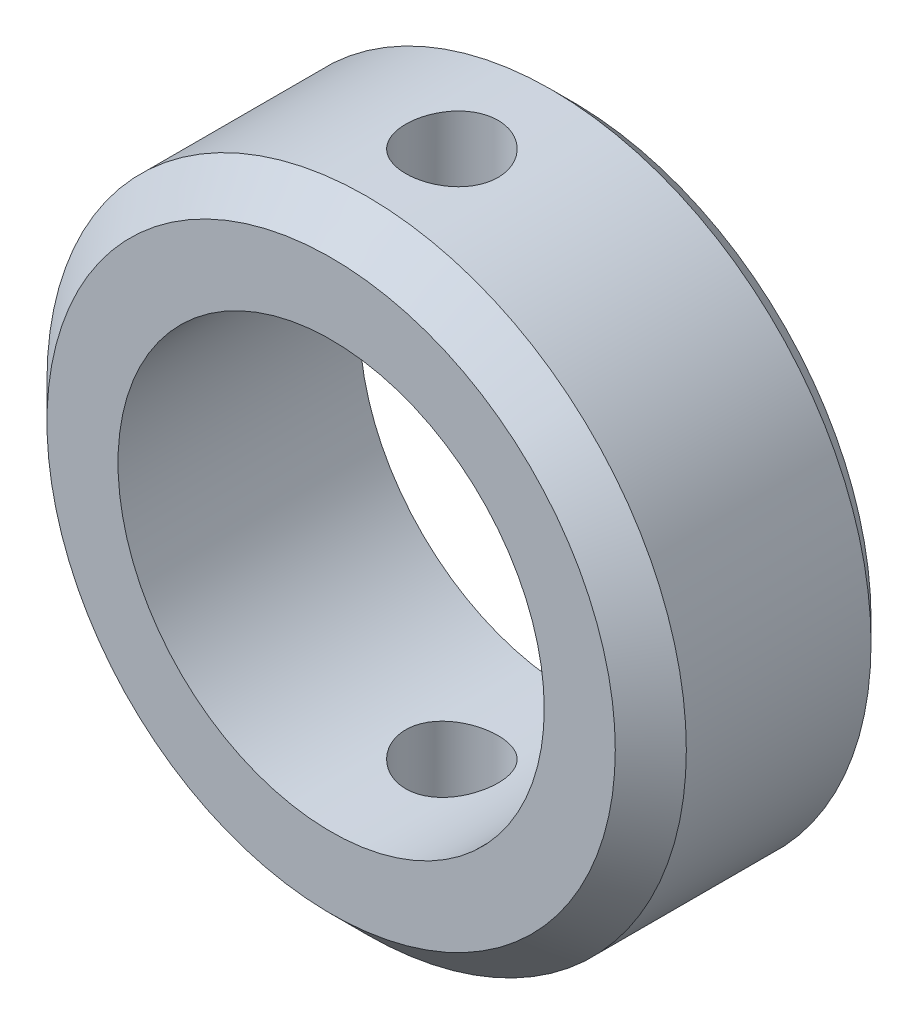
from build123d import *

# Parameters (mm, degrees)
SKETCH1_R               = 45
SKETCH1_R_2             = 30
BOSS_EXTRUDE1_DEPTH     = 34
CUT_EXTRUDE1_DEPTH      = 73.15261603
CUT_EXTRUDE1_DEPTH_BACK = 73.15261603
SKETCH3_R               = 6.5
CHAMFER1_SIZE           = 5
CHAMFER2_SIZE           = 3


with BuildPart() as part:
    # Sketch1 → Boss-Extrude1 (new body)
    with BuildSketch(Plane.XY):
        Circle(SKETCH1_R)
        Circle(SKETCH1_R_2, mode=Mode.SUBTRACT)
    extrude(amount=BOSS_EXTRUDE1_DEPTH)

    # Sketch3 → Cut-Extrude1 (cut, two sides: drawn at the far end of the back side and taken through both)
    with BuildSketch(Plane(origin=(0, 0, 0), x_dir=(1, 0, 0), z_dir=(0, 1, 0)).offset(-CUT_EXTRUDE1_DEPTH_BACK)):
        with Locations(Location((0, -17, 0), (0, 0, 270))):
            Circle(SKETCH3_R)
    extrude(amount=CUT_EXTRUDE1_DEPTH + CUT_EXTRUDE1_DEPTH_BACK, mode=Mode.SUBTRACT)

    # Chamfer1
    chamfer1_edges = [part.edges().sort_by_distance(p)[0] for p in [
        (-45, 0, 34),
    ]]
    chamfer(chamfer1_edges, length=CHAMFER1_SIZE)

    # Chamfer2
    chamfer2_edges = [part.edges().sort_by_distance(p)[0] for p in [
        (-45, 0, 0),
    ]]
    chamfer(chamfer2_edges, length=CHAMFER2_SIZE)


solid = part.part
